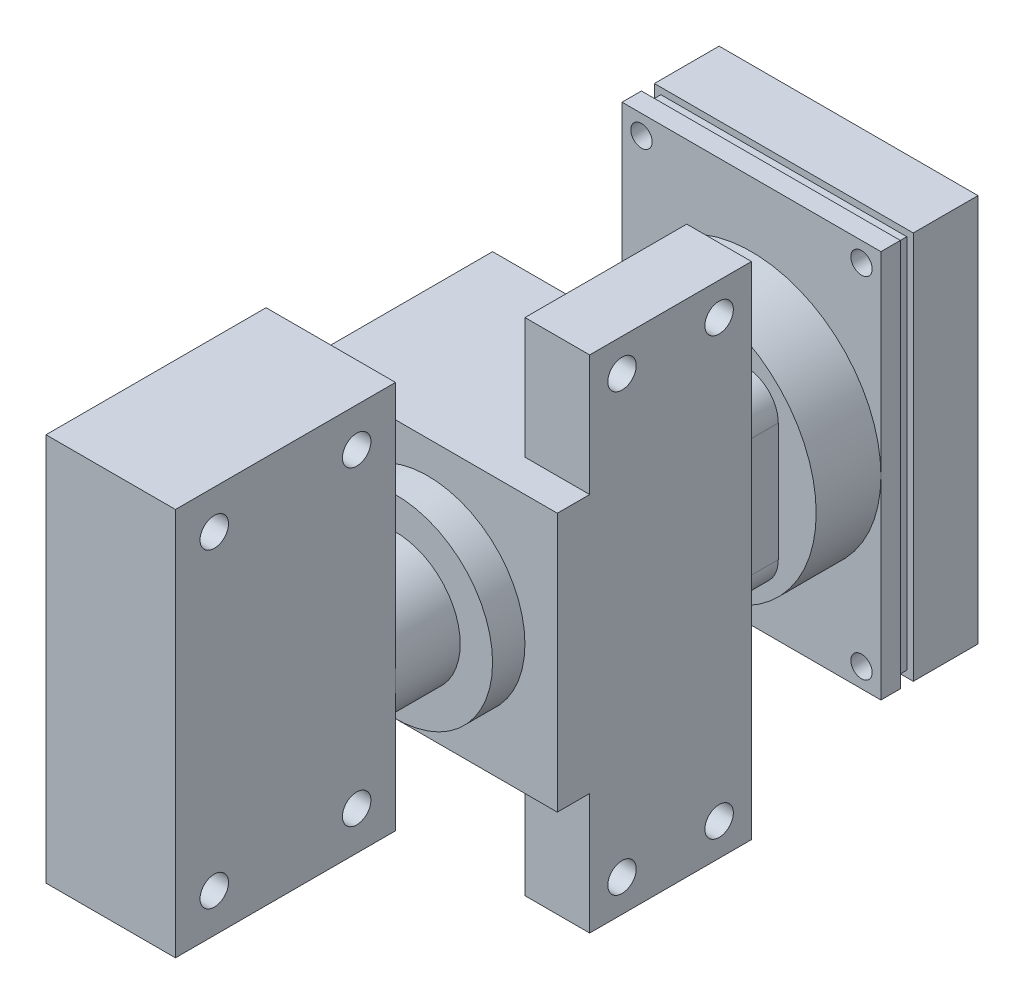
from build123d import *

# Parameters (mm, degrees)
SKETCH_1_W          = 40
SKETCH_1_H          = 60
EXTRUDE_1_DEPTH     = 10
SKETCH_2_W          = 38
SKETCH_2_H          = 58
EXTRUDE_2_DEPTH     = 2
SKETCH_3_W          = 40
SKETCH_3_H          = 60
EXTRUDE_3_DEPTH     = 3
SKETCH_4_R          = 20
EXTRUDE_4_DEPTH     = 10
EXTRUDE_5_DEPTH     = 10
SKETCH_6_R          = 1.65
CUT_EXTRUDE_1_DEPTH = 20
EXTRUDE_6_DEPTH     = 30
SKETCH_8_R          = 15
EXTRUDE_7_DEPTH     = 5
SKETCH_9_R          = 10
EXTRUDE_8_DEPTH     = 10
SKETCH_10_W         = 25
SKETCH_10_H         = 18.68197258
EXTRUDE_9_DEPTH     = 10
SKETCH_11_R         = 2.2
CUT_EXTRUDE_2_DEPTH = 10
SKETCH_12_W         = 20
SKETCH_12_H         = 60
EXTRUDE_10_DEPTH    = 34
SKETCH_13_R         = 2.2
CUT_EXTRUDE_3_DEPTH = 35


with BuildPart() as part:
    # 草图1 → 凸台-拉伸1 (new body)
    with BuildSketch(Plane.XY):
        Rectangle(SKETCH_1_W, SKETCH_1_H)
    extrude(amount=EXTRUDE_1_DEPTH)

    # 草图2 → 凸台-拉伸2 (add)
    with BuildSketch(Plane.XY.offset(10)):
        Rectangle(SKETCH_2_W, SKETCH_2_H)
    extrude(amount=EXTRUDE_2_DEPTH)

    # 草图3 → 凸台-拉伸3 (add)
    with BuildSketch(Plane.XY.offset(12)):
        Rectangle(SKETCH_3_W, SKETCH_3_H)
    extrude(amount=EXTRUDE_3_DEPTH)

    # 草图4 → 凸台-拉伸4 (add)
    with BuildSketch(Plane.XY.offset(15)):
        Circle(SKETCH_4_R)
    extrude(amount=EXTRUDE_4_DEPTH)

    # 草图5 → 凸台-拉伸5 (add)
    with BuildSketch(Plane.XY.offset(25)):
        with BuildLine():
            Line((9.142135624, -14.142135624), (-9.142135624, -14.142135624))
            ThreePointArc((-9.142135624, -14.142135624), (-12.67766953, -12.67766953), (-14.142135624, -9.142135624))
            Line((-14.142135624, -9.142135624), (-14.142135624, 9.142135624))
            ThreePointArc((-14.142135624, 9.142135624), (-12.67766953, 12.67766953), (-9.142135624, 14.142135624))
            Line((-9.142135624, 14.142135624), (9.142135624, 14.142135624))
            ThreePointArc((9.142135624, 14.142135624), (12.67766953, 12.67766953), (14.142135624, 9.142135624))
            Line((14.142135624, 9.142135624), (14.142135624, -9.142135624))
            ThreePointArc((14.142135624, -9.142135624), (12.67766953, -12.67766953), (9.142135624, -14.142135624))
        make_face()
    extrude(amount=EXTRUDE_5_DEPTH)

    # 草图6 → 切除-拉伸1 (cut)
    with BuildSketch(Plane(origin=(0, 0, 0), x_dir=(-1, 0, 0), z_dir=(0, 0, -1))):
        with Locations((17, 27)):
            Circle(SKETCH_6_R)
        with Locations((17, -27)):
            Circle(SKETCH_6_R)
        with Locations((-17, -27)):
            Circle(SKETCH_6_R)
        with Locations((-17, 27)):
            Circle(SKETCH_6_R)
    extrude(amount=-CUT_EXTRUDE_1_DEPTH, mode=Mode.SUBTRACT)

    # 草图7 → 凸台-拉伸6 (add)
    with BuildSketch(Plane.XY.offset(35)):
        Polygon((20, -20), (20, 20), (-20, 20), (-20, 10), (-30, 10), (-30, -20), align=None)
    extrude(amount=EXTRUDE_6_DEPTH)

    # 草图8 → 凸台-拉伸7 (add)
    with BuildSketch(Plane.XY.offset(65)):
        Circle(SKETCH_8_R)
    extrude(amount=EXTRUDE_7_DEPTH)

    # 草图9 → 凸台-拉伸8 (add)
    with BuildSketch(Plane.XY.offset(70)):
        Circle(SKETCH_9_R)
    extrude(amount=EXTRUDE_8_DEPTH)

    # 草图10 → 凸台-拉伸9 (add)
    with BuildSketch(Plane(origin=(20, 0, 0), x_dir=(0, 0, -1), z_dir=(1, 0, 0))):
        with Locations((-47.5, 29.34098629)):
            Rectangle(SKETCH_10_W, SKETCH_10_H)
        with Locations((-47.5, -29.34098629)):
            Rectangle(SKETCH_10_W, SKETCH_10_H)
    extrude(amount=-EXTRUDE_9_DEPTH)

    # 草图11 → 切除-拉伸2 (cut)
    with BuildSketch(Plane.ZY.offset(-10)):
        with Locations((55, 33.68197258)):
            Circle(SKETCH_11_R)
        with Locations((40, 33.68197258)):
            Circle(SKETCH_11_R)
        with Locations((40, -33.68197258)):
            Circle(SKETCH_11_R)
        with Locations((55, -33.68197258)):
            Circle(SKETCH_11_R)
    extrude(amount=-CUT_EXTRUDE_2_DEPTH, mode=Mode.SUBTRACT)

    # 草图12 → 凸台-拉伸10 (add)
    with BuildSketch(Plane.XY.offset(80)):
        with Locations((0, 10)):
            Rectangle(SKETCH_12_W, SKETCH_12_H)
    extrude(amount=EXTRUDE_10_DEPTH)

    # 草图13 → 切除-拉伸3 (cut)
    with BuildSketch(Plane.ZY.offset(10)):
        with Locations(Location((108, 34, 0), (0, 0, 270))):
            Circle(SKETCH_13_R)
        with Locations(Location((86, 34, 0), (0, 0, 270))):
            Circle(SKETCH_13_R)
        with Locations(Location((108, -14, 0), (0, 0, 270))):
            Circle(SKETCH_13_R)
        with Locations(Location((86, -14, 0), (0, 0, 270))):
            Circle(SKETCH_13_R)
    extrude(amount=-CUT_EXTRUDE_3_DEPTH, mode=Mode.SUBTRACT)


solid = part.part
